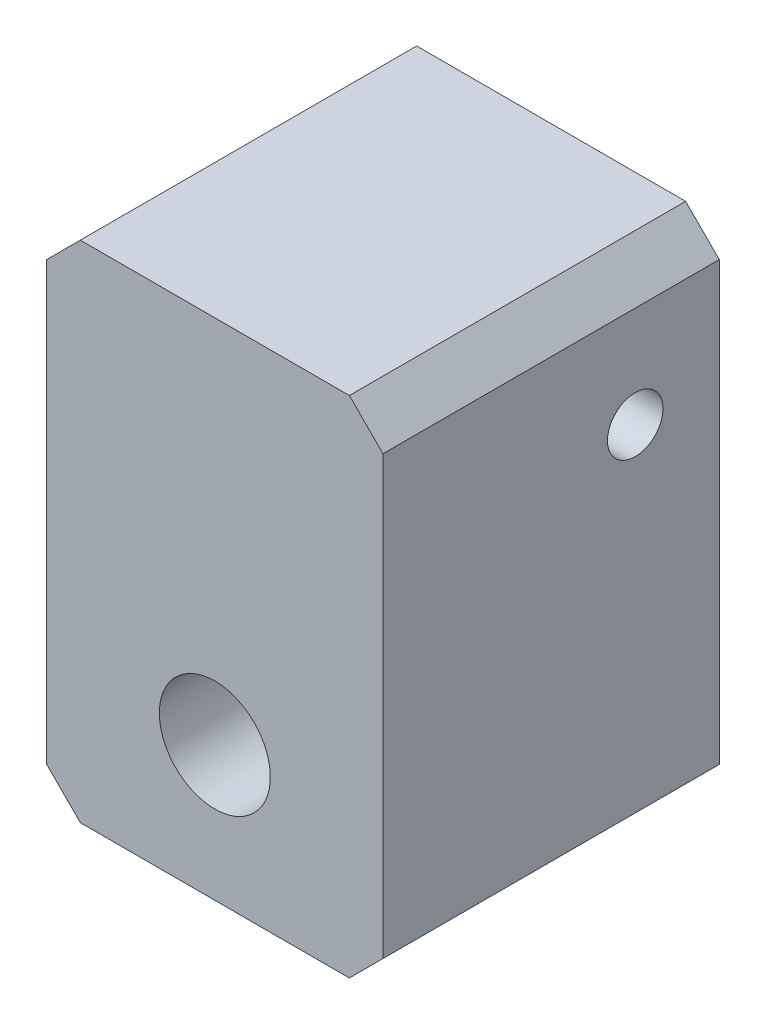
from build123d import *

# Parameters (mm, degrees)
SKETCH_1_W                = 20
SKETCH_1_H                = 30
EXTRUDE_1_DEPTH           = 20
HOLE_WIZARD_1_D           = 6.6
HOLE_WIZARD_1_CBORE_D     = 11
HOLE_WIZARD_1_CBORE_DEPTH = 6.8
HOLE_WIZARD_M4_1_D        = 3.3
CHAMFER_1_SIZE            = 2


with BuildPart() as part:
    # 草图1 → 凸台-拉伸1 (new body)
    with BuildSketch(Plane.XY):
        Rectangle(SKETCH_1_W, SKETCH_1_H)
    extrude(amount=EXTRUDE_1_DEPTH)

    # 打孔尺寸根据内六角圆柱头螺钉的类型1 (through all)
    with Locations(Plane(origin=(3.133596483, 10.907898158, 0), x_dir=(1, 0, 0), z_dir=(0, 0, -1))):
        with Locations((-3.133596483, 17.907898158)):
            CounterBoreHole(HOLE_WIZARD_1_D / 2, HOLE_WIZARD_1_CBORE_D / 2, HOLE_WIZARD_1_CBORE_DEPTH)

    # M4 螺纹孔1 (through all)
    with Locations(Plane.ZY.offset(10)):
        with Locations((5, 7)):
            Hole(HOLE_WIZARD_M4_1_D / 2)

    # 倒角1
    chamfer_1_edges = [part.edges().sort_by_distance(p)[0] for p in [
        (10, -15, 10),
        (-10, -15, 10),
        (-10, 15, 10),
        (10, 15, 10),
    ]]
    chamfer(chamfer_1_edges, length=CHAMFER_1_SIZE)


solid = part.part
